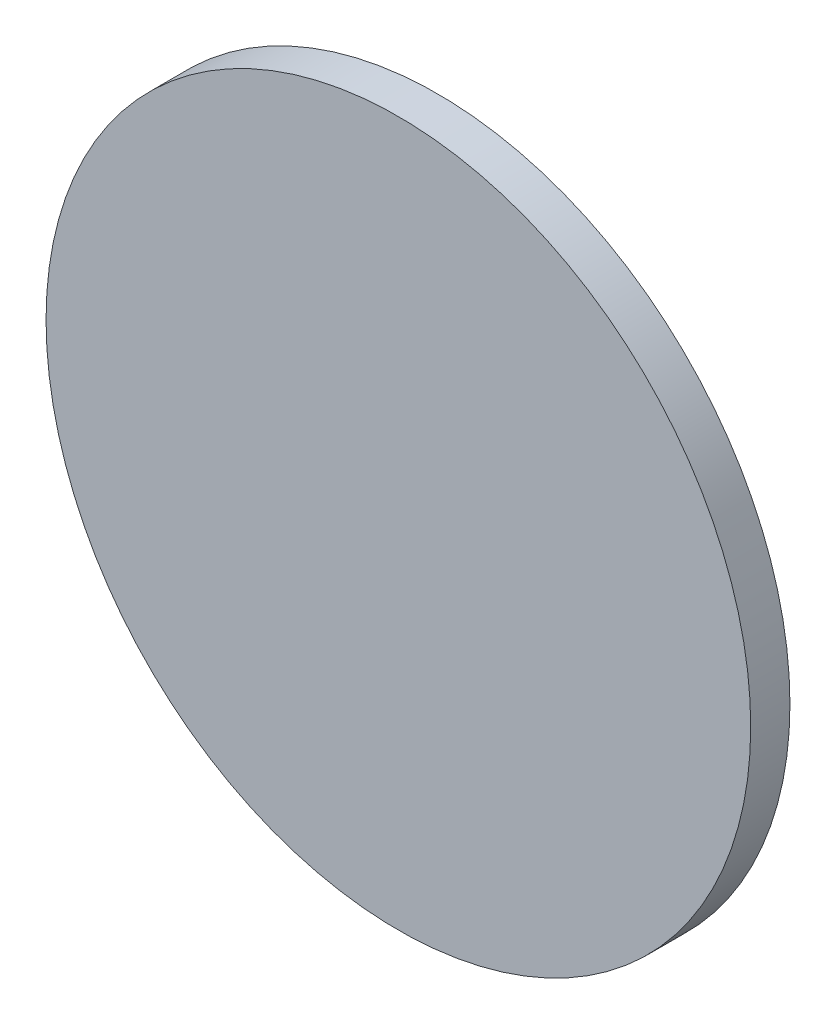
from build123d import *

# Parameters (mm, degrees)
SKETCH_1_R      = 26.95
EXTRUDE_1_DEPTH = 3


with BuildPart() as part:
    # 草图1 → 凸台-拉伸1 (new body)
    with BuildSketch(Plane.XY):
        Circle(SKETCH_1_R)
    extrude(amount=EXTRUDE_1_DEPTH)


solid = part.part
